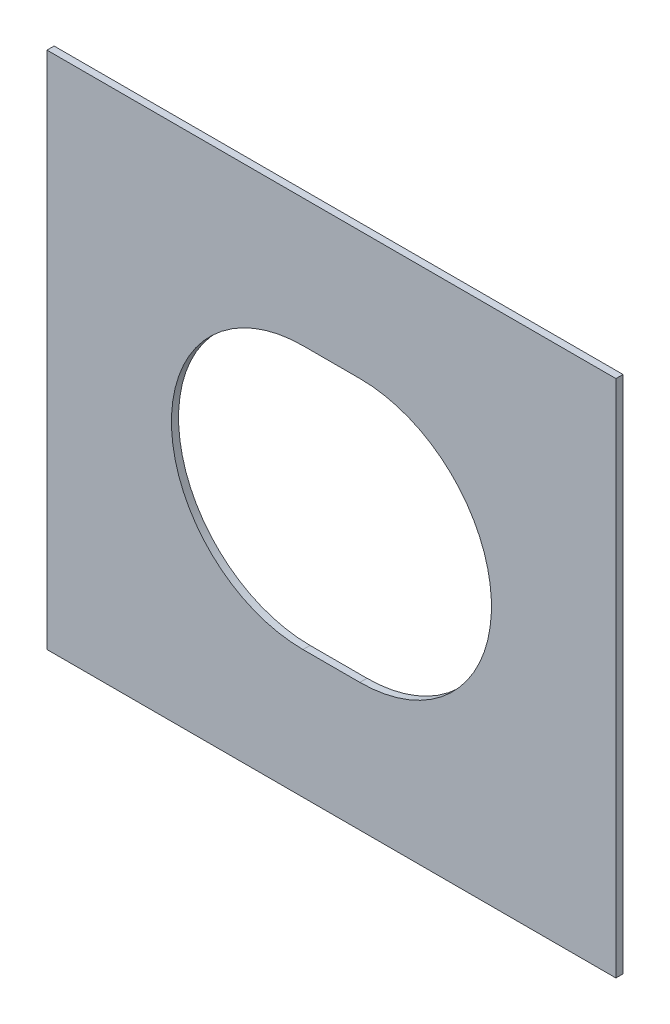
from build123d import *

# Parameters (mm, degrees)
SKETCH_1_W          = 400
SKETCH_1_H          = 365
EXTRUDE_1_DEPTH     = 5
CUT_EXTRUDE_3_DEPTH = 10


with BuildPart() as part:
    # 草图1 → 凸台-拉伸1 (new body)
    with BuildSketch(Plane.XY):
        with Locations((200, 182.5)):
            Rectangle(SKETCH_1_W, SKETCH_1_H)
    extrude(amount=EXTRUDE_1_DEPTH)

    # 草图4 → 切除-拉伸3 (cut)
    with BuildSketch(Plane.XY.offset(5)):
        with BuildLine():
            Line((180, 275), (220, 275))
            ThreePointArc((220, 275), (312.5, 182.5), (220, 90))
            Line((220, 90), (180, 90))
            ThreePointArc((180, 90), (87.5, 182.5), (180, 275))
        make_face()
    extrude(amount=-CUT_EXTRUDE_3_DEPTH, mode=Mode.SUBTRACT)


solid = part.part
